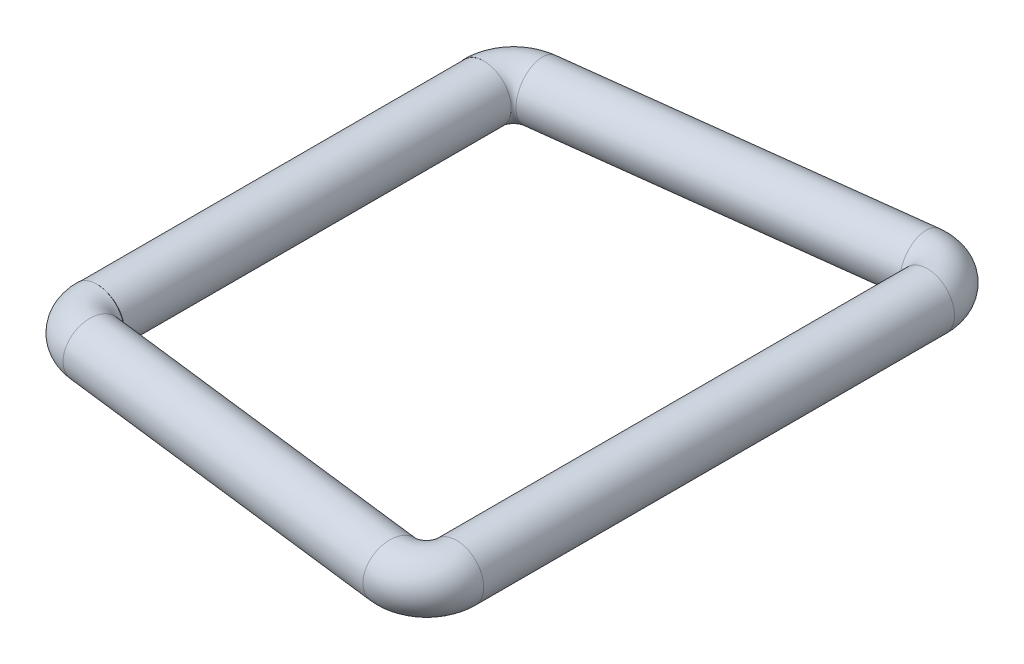
from build123d import *

# Parameters (mm, degrees)
EXTRUDE_1_DEPTH      = 8.65
EXTRUDE_1_DEPTH_BACK = 8.65
SKETCH_1_R           = 1
SKETCH_2_R           = 1
REVOLVE_1_ANGLE      = 97
SKETCH_3_R           = 1
REVOLVE_2_ANGLE      = 97
SKETCH_4_R           = 1
EXTRUDE_2_DEPTH      = 12.65745
SKETCH_5_R           = 1
EXTRUDE_3_DEPTH      = 12.65745
SKETCH_6_R           = 1
REVOLVE_3_ANGLE      = 83
SKETCH_7_R           = 1
REVOLVE_4_ANGLE      = 83
EXTRUDE_4_DEPTH      = 7.10745
EXTRUDE_4_DEPTH_BACK = 7.10745
SKETCH_8_R           = 1


with BuildPart() as part:
    # 草图1 → 凸台-拉伸1 (new, two sides: drawn at the far end of the back side and taken through both)
    with BuildSketch(Plane.XY.offset(-EXTRUDE_1_DEPTH_BACK)):
        with Locations((8.57, 0)):
            Circle(SKETCH_1_R)
    extrude(amount=EXTRUDE_1_DEPTH + EXTRUDE_1_DEPTH_BACK)

    # 草图2 → 旋转1 (revolve)
    with BuildSketch(Plane(origin=(0, 0, -8.65), x_dir=(-1, 0, 0), z_dir=(0, 0, -1))):
        with Locations(Location((-8.57, 0, 0), (0, 0, 180))):
            Circle(SKETCH_2_R)
    revolve(axis=Axis((7.47, 1, -8.65), (0, 1, 0)), revolution_arc=REVOLVE_1_ANGLE)

    # 草图3 → 旋转2 (revolve)
    with BuildSketch(Plane.XY.offset(8.65)):
        with Locations((8.57, 0)):
            Circle(SKETCH_3_R)
    revolve(axis=Axis((7.47, -1, 8.65), (0, -1, 0)), revolution_arc=REVOLVE_2_ANGLE)

    # 草图4 → 凸台-拉伸2 (add)
    with BuildSketch(Plane(origin=(8.405366736, 0, -1.032049264), x_dir=(0.12186934340514718, 0, 0.9925461516413221), z_dir=(-0.9925461516413221, 0, 0.12186934340514718))):
        with Locations(Location((-8.775160216, 0, 0), (0, 0, 180))):
            Circle(SKETCH_4_R)
    extrude(amount=EXTRUDE_2_DEPTH)

    # 草图5 → 凸台-拉伸3 (add)
    with BuildSketch(Plane(origin=(8.405366736, 0, 1.032049264), x_dir=(-0.12186934340514718, 0, 0.9925461516413221), z_dir=(-0.9925461516413221, 0, -0.12186934340514718))):
        with Locations((8.775160216, 0)):
            Circle(SKETCH_5_R)
    extrude(amount=EXTRUDE_3_DEPTH)

    # 草图6 → 旋转3 (revolve)
    with BuildSketch(Plane(origin=(-4.157736551, 0, 0.510505857), x_dir=(0.12186934340514717, 0, 0.9925461516413221), z_dir=(-0.9925461516413221, 0, 0.12186934340514717))):
        with Locations(Location((-8.775160216, 0, 0), (0, 0, 180))):
            Circle(SKETCH_6_R)
    revolve(axis=Axis((-5.093103287, 1, -7.107444879), (0, 1, 0)), revolution_arc=REVOLVE_3_ANGLE)

    # 草图7 → 旋转4 (revolve)
    with BuildSketch(Plane(origin=(-4.157736551, 0, -0.510505857), x_dir=(-0.12186934340514716, 0, 0.9925461516413221), z_dir=(-0.9925461516413221, 0, -0.12186934340514716))):
        with Locations((8.775160216, 0)):
            Circle(SKETCH_7_R)
    revolve(axis=Axis((-5.093103287, -1, 7.107444879), (0, -1, 0)), revolution_arc=REVOLVE_4_ANGLE)

    # 草图8 → 凸台-拉伸4 (add, two sides: drawn at the far end of the back side and taken through both)
    with BuildSketch(Plane.XY.offset(-EXTRUDE_4_DEPTH_BACK)):
        with Locations(Location((-6.177315, 0, 0), (0, 0, 90.452305782))):
            Circle(SKETCH_8_R)
    extrude(amount=EXTRUDE_4_DEPTH + EXTRUDE_4_DEPTH_BACK)


solid = part.part
